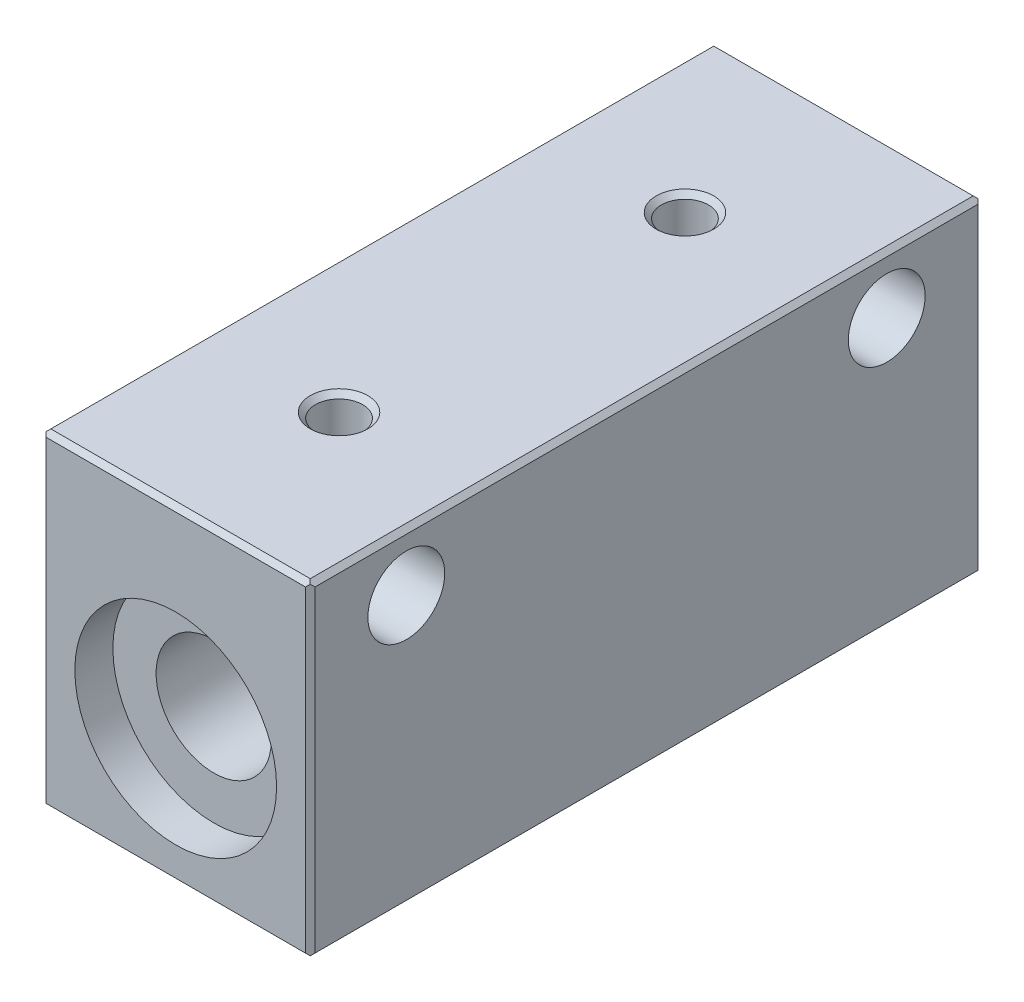
from build123d import *

# Parameters (mm, degrees)
EXTRUDE_1_DEPTH          = 14
EXTRUDE_1_DEPTH_BACK     = 14
SKETCH_3_W               = 6
SKETCH_3_H               = 4
SKETCH_4_W               = 6
SKETCH_4_H               = 4
CUT_EXTRUDE_1_DEPTH      = 35
CUT_EXTRUDE_1_DEPTH_BACK = 35
SKETCH_9_W               = 32
SKETCH_9_H               = 38
CUT_EXTRUDE_2_DEPTH      = 34
CUT_EXTRUDE_2_DEPTH_BACK = 34
SKETCH_10_W              = 32
SKETCH_10_H              = 74


with BuildPart() as part:
    # 草图1 → 凸台-拉伸1 (new, two sides: drawn at the far end of the back side and taken through both)
    with BuildSketch(Plane(origin=(0, 0, 0), x_dir=(0, 0, -1), z_dir=(1, 0, 0)).offset(-EXTRUDE_1_DEPTH_BACK)):
        Polygon((-35, -13.5), (-34.5, -14), (34.5, -14), (35, -13.5), (35, 19.5), (34.5, 20), (-34.5, 20), (-35, 19.5), align=None)
    extrude(amount=EXTRUDE_1_DEPTH + EXTRUDE_1_DEPTH_BACK)

    # 草图2 → 切除-旋转1 (revolve, cut)
    with BuildSketch(Plane(origin=(0, 0, 0), x_dir=(0, 0, -1), z_dir=(1, 0, 0)), mode=Mode.PRIVATE) as cut_revolve_1_sk:
        Polygon((-35, 0), (-35, 10.5), (-31.04, 10.5), (-31.04, 6), (31.04, 6), (31.04, 10.5), (35, 10.5), (35, 0), align=None)
    revolve(cut_revolve_1_sk.sketch.rotate(Axis((0, 0, -35), (0, 0, 1)), 270), axis=Axis((0, 0, -35), (0, 0, 1)), mode=Mode.SUBTRACT)

    # 草图3 → 切除-旋转2 (revolve, cut)
    with BuildSketch(Plane.XY.offset(25), mode=Mode.PRIVATE) as cut_revolve_2_sk:
        with Locations((11, 16)):
            Rectangle(SKETCH_3_W, SKETCH_3_H)
    revolve(cut_revolve_2_sk.sketch.rotate(Axis((14, 14, 25), (-1, 0, 0)), 270), axis=Axis((14, 14, 25), (-1, 0, 0)), mode=Mode.SUBTRACT)

    # 草图4 → 切除-旋转3 (revolve, cut)
    with BuildSketch(Plane.XY.offset(-25), mode=Mode.PRIVATE) as cut_revolve_3_sk:
        with Locations((11, 16)):
            Rectangle(SKETCH_4_W, SKETCH_4_H)
    revolve(cut_revolve_3_sk.sketch.rotate(Axis((14, 14, -25), (-1, 0, 0)), 270), axis=Axis((14, 14, -25), (-1, 0, 0)), mode=Mode.SUBTRACT)

    # 草图5 → 切除-旋转4 (revolve, cut)
    with BuildSketch(Plane(origin=(0, 0, 0), x_dir=(0, 0, -1), z_dir=(1, 0, 0)), mode=Mode.PRIVATE) as cut_revolve_4_sk:
        Polygon((18, 20), (21, 20), (20.4585, 19.4585), (20.4585, 10.92), (18, 10.92), align=None)
    revolve(cut_revolve_4_sk.sketch.rotate(Axis((0, 10.92, -18), (0, 1, 0)), 180), axis=Axis((0, 10.92, -18), (0, 1, 0)), mode=Mode.SUBTRACT)

    # 草图6 → 切除-旋转5 (revolve, cut)
    with BuildSketch(Plane(origin=(0, 0, 0), x_dir=(0, 0, -1), z_dir=(1, 0, 0)), mode=Mode.PRIVATE) as cut_revolve_5_sk:
        Polygon((-18, 20), (-15, 20), (-15.5415, 19.4585), (-15.5415, 10.92), (-18, 10.92), align=None)
    revolve(cut_revolve_5_sk.sketch.rotate(Axis((0, 10.92, 18), (0, 1, 0)), 180), axis=Axis((0, 10.92, 18), (0, 1, 0)), mode=Mode.SUBTRACT)

    # 草图7 → 切除-旋转6 (revolve, cut)
    with BuildSketch(Plane.XY.offset(-25), mode=Mode.PRIVATE) as cut_revolve_6_sk:
        Polygon((-14, 14), (-14, 16.5), (-13.567, 16.067), (8, 16.067), (8, 14), align=None)
    revolve(cut_revolve_6_sk.sketch.rotate(Axis((8, 14, -25), (-1, 0, 0)), 270), axis=Axis((8, 14, -25), (-1, 0, 0)), mode=Mode.SUBTRACT)

    # 草图8 → 切除-旋转7 (revolve, cut)
    with BuildSketch(Plane.XY.offset(25), mode=Mode.PRIVATE) as cut_revolve_7_sk:
        Polygon((-14, 14), (-14, 16.5), (-13.567, 16.067), (8, 16.067), (8, 14), align=None)
    revolve(cut_revolve_7_sk.sketch.rotate(Axis((8, 14, 25), (-1, 0, 0)), 270), axis=Axis((8, 14, 25), (-1, 0, 0)), mode=Mode.SUBTRACT)

    # 草图9 → 切除-拉伸1 (cut, two sides: drawn at the far end of the back side and taken through both)
    with BuildSketch(Plane.XY.offset(-CUT_EXTRUDE_1_DEPTH_BACK)):
        with Locations((0, 3)):
            Rectangle(SKETCH_9_W, SKETCH_9_H)
        Polygon((-14, -13.5), (-13.5, -14), (13.5, -14), (14, -13.5), (14, 19.5), (13.5, 20), (-13.5, 20), (-14, 19.5), align=None, mode=Mode.SUBTRACT)
    extrude(amount=CUT_EXTRUDE_1_DEPTH + CUT_EXTRUDE_1_DEPTH_BACK, mode=Mode.SUBTRACT)

    # 草图10 → 切除-拉伸2 (cut, two sides: drawn at the far end of the back side and taken through both)
    with BuildSketch(Plane(origin=(0, 0, 0), x_dir=(1, 0, 0), z_dir=(0, 1, 0)).offset(-CUT_EXTRUDE_2_DEPTH_BACK)):
        Rectangle(SKETCH_10_W, SKETCH_10_H)
        Polygon((-14, -34.5), (-13.5, -35), (13.5, -35), (14, -34.5), (14, 34.5), (13.5, 35), (-13.5, 35), (-14, 34.5), align=None, mode=Mode.SUBTRACT)
    extrude(amount=CUT_EXTRUDE_2_DEPTH + CUT_EXTRUDE_2_DEPTH_BACK, mode=Mode.SUBTRACT)


solid = part.part
